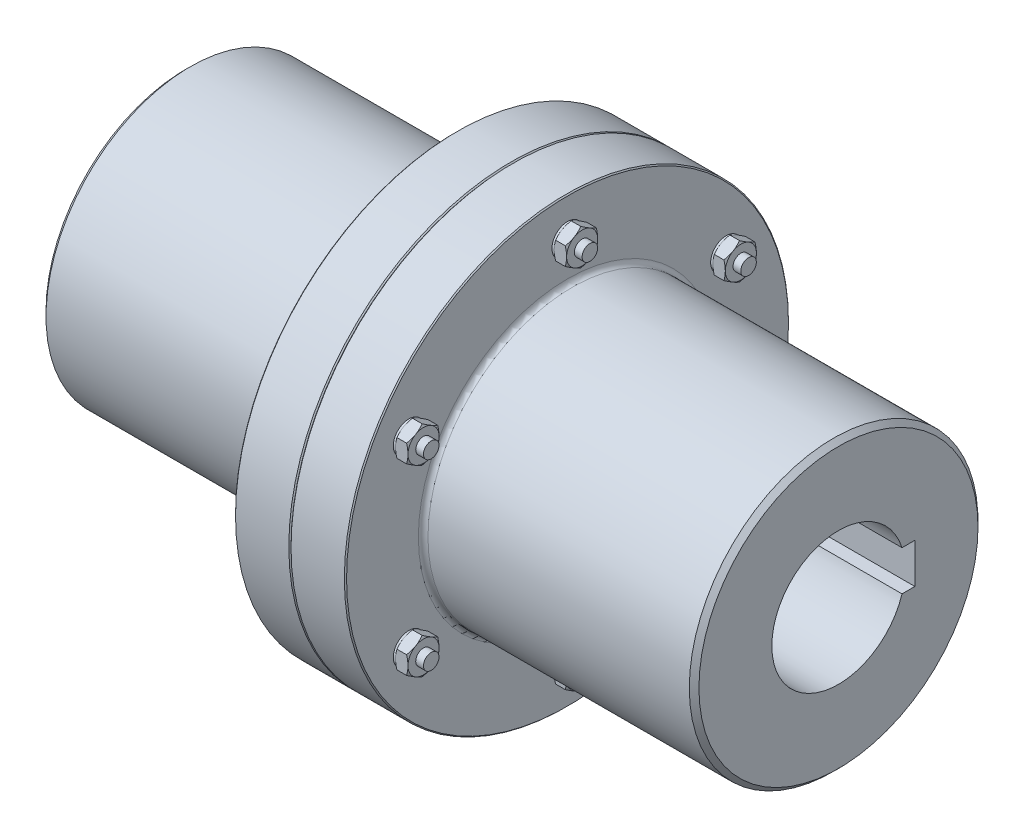
from build123d import *

# Parameters (mm, degrees)
CHAMFER1_SIZE                  = 2.166666667
CHAMFER2_SIZE                  = 0.5
FILLET1_R                      = 1
SKETCH15_R                     = 37.5
CUT_EXTRUDE5_DEPTH             = 204.982842416
CUT_EXTRUDE7_DEPTH             = 204.982842416
SKETCH16_R                     = 30
CUT_EXTRUDE6_DEPTH             = 204.982842416
CUT_EXTRUDE10_DEPTH            = 204.982842416
CHAMFER3_SIZE                  = 0.5
CHAMFER4_SIZE                  = 2.166666667
FILLET2_R                      = 2.166666667
SKETCH6_R                      = 3.5
CUT_EXTRUDE1_DEPTH             = 50
CHAMFER5_SIZE                  = 0.2
CHAMFER6_SIZE                  = 0.2
CIRPATTERN1_COUNT              = 6
CHAMFER5_OF_CIRPATTERN1_SIZE   = 0.2
CHAMFER6_OF_CIRPATTERN1_SIZE   = 0.2
SKETCH7_W                      = 60.08
SKETCH7_H                      = 3.5
BOSS_EXTRUDE1_DEPTH            = 5.6
SKETCH9_R                      = 10.5
SKETCH9_R_2                    = 7
CUT_EXTRUDE2_DEPTH             = 1
CUT_EXTRUDE2_DRAFT             = -60
SKETCH10_R                     = 7
BOSS_EXTRUDE2_DEPTH            = 1
BOSS_EXTRUDE3_DEPTH            = 5.6
SKETCH12_R                     = 10.5
SKETCH12_R_2                   = 7
CUT_EXTRUDE3_DEPTH             = 1
CUT_EXTRUDE3_DRAFT             = -60
SKETCH13_R                     = 10.5
SKETCH13_R_2                   = 7
CUT_EXTRUDE4_DEPTH             = 1
CUT_EXTRUDE4_DRAFT             = -60
CIRPATTERN3_COUNT              = 6
CIRPATTERN3_COPY_1_SKETCH_R    = 10.5
CIRPATTERN3_COPY_1_SKETCH_R_2  = 7
CIRPATTERN3_COPY_1_DEPTH       = 1
CIRPATTERN3_COPY_1_DRAFT       = -60
CIRPATTERN3_COPY_2_SKETCH_R    = 10.5
CIRPATTERN3_COPY_2_SKETCH_R_2  = 7
CIRPATTERN3_COPY_2_DEPTH       = 1
CIRPATTERN3_COPY_2_DRAFT       = -60
CIRPATTERN3_COPY_3_SKETCH_R    = 10.5
CIRPATTERN3_COPY_3_SKETCH_R_2  = 7
CIRPATTERN3_COPY_3_DEPTH       = 1
CIRPATTERN3_COPY_3_DRAFT       = -60
CIRPATTERN3_COPY_4_SKETCH_R    = 10.5
CIRPATTERN3_COPY_4_SKETCH_R_2  = 7
CIRPATTERN3_COPY_4_DEPTH       = 1
CIRPATTERN3_COPY_4_DRAFT       = -60
CIRPATTERN3_COPY_5_SKETCH_R    = 10.5
CIRPATTERN3_COPY_5_SKETCH_R_2  = 7
CIRPATTERN3_COPY_5_DEPTH       = 1
CIRPATTERN3_COPY_5_DRAFT       = -60
CIRPATTERN3_COPY_6_SKETCH_R    = 10.5
CIRPATTERN3_COPY_6_SKETCH_R_2  = 7
CIRPATTERN3_COPY_6_DEPTH       = 1
CIRPATTERN3_COPY_6_DRAFT       = -60
CIRPATTERN3_COPY_7_SKETCH_R    = 10.5
CIRPATTERN3_COPY_7_SKETCH_R_2  = 7
CIRPATTERN3_COPY_7_DEPTH       = 1
CIRPATTERN3_COPY_7_DRAFT       = -60
CIRPATTERN3_COPY_8_SKETCH_R    = 10.5
CIRPATTERN3_COPY_8_SKETCH_R_2  = 7
CIRPATTERN3_COPY_8_DEPTH       = 1
CIRPATTERN3_COPY_8_DRAFT       = -60
CIRPATTERN3_COPY_9_SKETCH_R    = 10.5
CIRPATTERN3_COPY_9_SKETCH_R_2  = 7
CIRPATTERN3_COPY_9_DEPTH       = 1
CIRPATTERN3_COPY_9_DRAFT       = -60
CIRPATTERN3_COPY_10_SKETCH_R   = 10.5
CIRPATTERN3_COPY_10_SKETCH_R_2 = 7
CIRPATTERN3_COPY_10_DEPTH      = 1
CIRPATTERN3_COPY_10_DRAFT      = -60
CIRPATTERN3_COPY_11_SKETCH_R   = 10.5
CIRPATTERN3_COPY_11_SKETCH_R_2 = 7
CIRPATTERN3_COPY_11_DEPTH      = 1
CIRPATTERN3_COPY_11_DRAFT      = -60
CIRPATTERN3_COPY_12_SKETCH_R   = 10.5
CIRPATTERN3_COPY_12_SKETCH_R_2 = 7
CIRPATTERN3_COPY_12_DEPTH      = 1
CIRPATTERN3_COPY_12_DRAFT      = -60
CIRPATTERN3_COPY_13_SKETCH_R   = 10.5
CIRPATTERN3_COPY_13_SKETCH_R_2 = 7
CIRPATTERN3_COPY_13_DEPTH      = 1
CIRPATTERN3_COPY_13_DRAFT      = -60
CIRPATTERN3_COPY_14_SKETCH_R   = 10.5
CIRPATTERN3_COPY_14_SKETCH_R_2 = 7
CIRPATTERN3_COPY_14_DEPTH      = 1
CIRPATTERN3_COPY_14_DRAFT      = -60
CIRPATTERN3_COPY_15_SKETCH_R   = 10.5
CIRPATTERN3_COPY_15_SKETCH_R_2 = 7
CIRPATTERN3_COPY_15_DEPTH      = 1
CIRPATTERN3_COPY_15_DRAFT      = -60


with BuildPart() as part:
    # Sketch2 → Revolve1 (revolve)
    with BuildSketch(Plane.XY, mode=Mode.PRIVATE) as revolve1_sk:
        Polygon((-147, 65), (-147, 0), (-5, 0), (-5, 70), (0, 70), (0, 100), (-25, 100), (-25, 65), align=None)
    revolve(revolve1_sk.sketch.rotate(Axis((-147, 0, 0), (1, 0, 0)), 90), axis=Axis((-147, 0, 0), (1, 0, 0)))

    # Chamfer1
    chamfer1_edges = [part.edges().sort_by_distance(p)[0] for p in [
        (-147, 0, -65),
    ]]
    chamfer(chamfer1_edges, length=CHAMFER1_SIZE)

    # Chamfer2
    chamfer2_edges = [part.edges().sort_by_distance(p)[0] for p in [
        (-25, 0, -100),
        (0, 0, -100),
    ]]
    chamfer(chamfer2_edges, length=CHAMFER2_SIZE)

    # Fillet1
    fillet1_edges = [part.edges().sort_by_distance(p)[0] for p in [
        (-25, 0, -65),
    ]]
    fillet(fillet1_edges, radius=FILLET1_R)

    # Sketch15 → Cut-Extrude5 (cut, through all)
    with BuildSketch(Plane(origin=(0, 0, 0), x_dir=(0, 0, -1), z_dir=(1, 0, 0))):
        Circle(SKETCH15_R)
    extrude(amount=-CUT_EXTRUDE5_DEPTH, mode=Mode.SUBTRACT)

    # Sketch20 → Cut-Extrude7 (cut, through all)
    with BuildSketch(Plane(origin=(0, 0, 0), x_dir=(0, 0, -1), z_dir=(1, 0, 0))):
        with BuildLine():
            Line((42.4, -10), (42.4, 10))
            Line((42.4, 10), (36.142080737, 10))
            ThreePointArc((36.142080737, 10), (37.158969493, 5.045888047), (37.5, 0))
            ThreePointArc((37.5, 0), (37.158969493, -5.045888047), (36.142080737, -10))
            Line((36.142080737, -10), (42.4, -10))
        make_face()
    extrude(amount=-CUT_EXTRUDE7_DEPTH, mode=Mode.SUBTRACT)


with BuildPart() as body_2:
    # Sketch3 → Revolve2 (revolve)
    with BuildSketch(Plane.XY, mode=Mode.PRIVATE) as revolve2_sk:
        Polygon((25, 100), (0, 100), (0, 70), (5, 70), (5, 0), (147, 0), (147, 30), (147, 65), (25, 65), align=None)
    revolve(revolve2_sk.sketch.rotate(Axis((-147, 0, 0), (1, 0, 0)), 270), axis=Axis((-147, 0, 0), (1, 0, 0)))

    # Sketch16 → Cut-Extrude6 (cut, through all)
    with BuildSketch(Plane(origin=(0, 0, 0), x_dir=(0, 0, -1), z_dir=(1, 0, 0))):
        Circle(SKETCH16_R)
    extrude(amount=CUT_EXTRUDE6_DEPTH, mode=Mode.SUBTRACT)

    # Sketch24 → Cut-Extrude10 (cut, through all)
    with BuildSketch(Plane(origin=(0, 0, 0), x_dir=(0, 0, -1), z_dir=(1, 0, 0))):
        with BuildLine():
            Line((34.4, -9), (34.4, 9))
            Line((34.4, 9), (28.618176043, 9))
            ThreePointArc((28.618176043, 9), (29.652531774, 4.552730978), (30, 0))
            ThreePointArc((30, 0), (29.652531774, -4.552730978), (28.618176043, -9))
            Line((28.618176043, -9), (34.4, -9))
        make_face()
    extrude(amount=CUT_EXTRUDE10_DEPTH, mode=Mode.SUBTRACT)

    # Chamfer3
    chamfer3_edges = [body_2.edges().sort_by_distance(p)[0] for p in [
        (25, 0, 100),
        (0, 0, 100),
    ]]
    chamfer(chamfer3_edges, length=CHAMFER3_SIZE)

    # Chamfer4
    chamfer4_edges = [body_2.edges().sort_by_distance(p)[0] for p in [
        (147, 0, 65),
    ]]
    chamfer(chamfer4_edges, length=CHAMFER4_SIZE)

    # Fillet2
    fillet2_edges = [body_2.edges().sort_by_distance(p)[0] for p in [
        (25, 0, 65),
    ]]
    fillet(fillet2_edges, radius=FILLET2_R)


with BuildPart() as cut_extrude1_tool:
    # Sketch6 → Cut-Extrude1 (new body)
    with BuildSketch(Plane.ZY.offset(25)):
        with Locations((0, 82.5)):
            Circle(SKETCH6_R)
    cut_extrude1 = extrude(amount=-CUT_EXTRUDE1_DEPTH)


with BuildPart() as part_1:
    add(part.part)

    # Cut-Extrude1: cut by cut_extrude1_tool
    add(cut_extrude1_tool.part, mode=Mode.SUBTRACT)

    # Chamfer5
    chamfer5_edges = [part_1.edges().sort_by_distance(p)[0] for p in [
        (-25, 82.5, -3.5),
    ]]
    chamfer(chamfer5_edges, length=CHAMFER5_SIZE)


with BuildPart() as body_2_1:
    add(body_2.part)

    # Cut-Extrude1: cut by cut_extrude1_tool
    add(cut_extrude1_tool.part, mode=Mode.SUBTRACT)

    # Chamfer6
    chamfer6_edges = [body_2_1.edges().sort_by_distance(p)[0] for p in [
        (25, 82.5, -3.5),
    ]]
    chamfer(chamfer6_edges, length=CHAMFER6_SIZE)


with BuildPart() as cirpattern1_tool:
    # CirPattern1: Cut-Extrude1 ×6 about axis
    cirpattern1_axis = Axis((0, 0, 0), (1, 0, 0))
    for i in range(1, CIRPATTERN1_COUNT):
        add(cut_extrude1.rotate(cirpattern1_axis, i * 360 / CIRPATTERN1_COUNT))


with BuildPart() as part_2:
    add(part_1.part)

    # CirPattern1: cut by cirpattern1_tool
    add(cirpattern1_tool.part, mode=Mode.SUBTRACT)

    # Chamfer5 of CirPattern1
    chamfer5_of_cirpattern1_edges = [part_2.edges().sort_by_distance(p)[0] for p in [
        (-25, 44.281088913, 69.697095812),
        (-25, -38.218911087, 73.197095812),
        (-25, -82.5, 3.5),
        (-25, -44.281088913, -69.697095812),
        (-25, 38.218911087, -73.197095812),
    ]]
    chamfer(chamfer5_of_cirpattern1_edges, length=CHAMFER5_OF_CIRPATTERN1_SIZE)



with BuildPart() as body_2_2:
    add(body_2_1.part)

    # CirPattern1: cut by cirpattern1_tool
    add(cirpattern1_tool.part, mode=Mode.SUBTRACT)

    # Chamfer6 of CirPattern1
    chamfer6_of_cirpattern1_edges = [body_2_2.edges().sort_by_distance(p)[0] for p in [
        (25, 44.281088913, 69.697095812),
        (25, -38.218911087, 73.197095812),
        (25, -82.5, 3.5),
        (25, -44.281088913, -69.697095812),
        (25, 38.218911087, -73.197095812),
    ]]
    chamfer(chamfer6_of_cirpattern1_edges, length=CHAMFER6_OF_CIRPATTERN1_SIZE)


with BuildPart() as part_3:
    add(part_2.part)

    add(body_2_2.part)  # Revolve3 merges body 2
    # Sketch7 → Revolve3 (revolve)
    with BuildSketch(Plane.XY, mode=Mode.PRIVATE) as revolve3_sk:
        with Locations((5.04, 84.25)):
            Rectangle(SKETCH7_W, SKETCH7_H)
    revolve3 = revolve(revolve3_sk.sketch.rotate(Axis((35.08, 82.5, 0), (-1, 0, 0)), 90), axis=Axis((35.08, 82.5, 0), (-1, 0, 0)))

    # Sketch8 → Boss-Extrude1 (add)
    with BuildSketch(Plane.ZY.offset(25)):
        Polygon((0, 90.582903769), (-7, 86.541451884), (-7, 78.458548116), (0, 74.417096231), (7, 78.458548116), (7, 86.541451884), align=None)
    boss_extrude1 = extrude(amount=BOSS_EXTRUDE1_DEPTH)


with BuildPart() as cut_extrude2_tool:
    # Sketch9 → Cut-Extrude2 (with draft: the straight prism first)
    with BuildSketch(Plane.ZY.offset(30.6)):
        with Locations((0, 82.5)):
            Circle(SKETCH9_R)
        with Locations((0, 82.5)):
            Circle(SKETCH9_R_2, mode=Mode.SUBTRACT)
    extrude(amount=-CUT_EXTRUDE2_DEPTH)
    # Cut-Extrude2: the draft: its side faces are tilted about the plane it starts from
    cut_extrude2_sides = [cut_extrude2_tool.faces().sort_by_distance(p)[0] for p in [
        (-30.1, 82.5, -10.5),
        (-30.1, 82.5, -7),
    ]]
    draft(cut_extrude2_sides, Plane.ZY.offset(30.6), CUT_EXTRUDE2_DRAFT)


with BuildPart() as part_4:
    add(part_3.part)

    # Cut-Extrude2: cut by cut_extrude2_tool
    add(cut_extrude2_tool.part, mode=Mode.SUBTRACT)

    # Sketch10 → Boss-Extrude2 (add)
    with BuildSketch(Plane(origin=(25, 0, 0), x_dir=(0, 0, -1), z_dir=(1, 0, 0))):
        with Locations(Location((0, 82.5, 0), (0, 0, 180))):
            Circle(SKETCH10_R)
    boss_extrude2 = extrude(amount=BOSS_EXTRUDE2_DEPTH)

    # Sketch11 → Boss-Extrude3 (add)
    with BuildSketch(Plane(origin=(26, 0, 0), x_dir=(0, 0, -1), z_dir=(1, 0, 0))):
        Polygon((7, 86.541451884), (0, 90.582903769), (-7, 86.541451884), (-7, 78.458548116), (0, 74.417096231), (7, 78.458548116), align=None)
    boss_extrude3 = extrude(amount=BOSS_EXTRUDE3_DEPTH)


with BuildPart() as cut_extrude3_tool:
    # Sketch12 → Cut-Extrude3 (with draft: the straight prism first)
    with BuildSketch(Plane(origin=(31.6, 0, 0), x_dir=(0, 0, -1), z_dir=(1, 0, 0))):
        with Locations((0, 82.5)):
            Circle(SKETCH12_R)
        with Locations(Location((0, 82.5, 0), (0, 0, 180))):
            Circle(SKETCH12_R_2, mode=Mode.SUBTRACT)
    extrude(amount=-CUT_EXTRUDE3_DEPTH)
    # Cut-Extrude3: the draft: its side faces are tilted about the plane it starts from
    cut_extrude3_sides = [cut_extrude3_tool.faces().sort_by_distance(p)[0] for p in [
        (31.1, 82.5, 10.5),
        (31.1, 82.5, -7),
    ]]
    draft(cut_extrude3_sides, Plane(origin=(31.6, 0, 0), x_dir=(0, 0, -1), z_dir=(1, 0, 0)), CUT_EXTRUDE3_DRAFT)


with BuildPart() as part_5:
    add(part_4.part)

    # Cut-Extrude3: cut by cut_extrude3_tool
    add(cut_extrude3_tool.part, mode=Mode.SUBTRACT)


with BuildPart() as cut_extrude4_tool:
    # Sketch13 → Cut-Extrude4 (with draft: the straight prism first)
    with BuildSketch(Plane.ZY.offset(-26)):
        with Locations((0, 82.5)):
            Circle(SKETCH13_R)
        with Locations((0, 82.5)):
            Circle(SKETCH13_R_2, mode=Mode.SUBTRACT)
    extrude(amount=-CUT_EXTRUDE4_DEPTH)
    # Cut-Extrude4: the draft: its side faces are tilted about the plane it starts from
    cut_extrude4_sides = [cut_extrude4_tool.faces().sort_by_distance(p)[0] for p in [
        (26.5, 82.5, -10.5),
        (26.5, 82.5, -7),
    ]]
    draft(cut_extrude4_sides, Plane.ZY.offset(-26), CUT_EXTRUDE4_DRAFT)


with BuildPart() as part_6:
    add(part_5.part)

    # Cut-Extrude4: cut by cut_extrude4_tool
    add(cut_extrude4_tool.part, mode=Mode.SUBTRACT)

    # CirPattern3: Revolve3, Boss-Extrude1, Boss-Extrude2, Boss-Extrude3 ×6 about axis
    cirpattern3_axis = Axis((0, 0, 0), (1, 0, 0))
    add([revolve3.rotate(cirpattern3_axis, i * 360 / CIRPATTERN3_COUNT) for i in range(1, CIRPATTERN3_COUNT)])
    add([boss_extrude1.rotate(cirpattern3_axis, i * 360 / CIRPATTERN3_COUNT) for i in range(1, CIRPATTERN3_COUNT)])
    add([boss_extrude2.rotate(cirpattern3_axis, i * 360 / CIRPATTERN3_COUNT) for i in range(1, CIRPATTERN3_COUNT)])
    add([boss_extrude3.rotate(cirpattern3_axis, i * 360 / CIRPATTERN3_COUNT) for i in range(1, CIRPATTERN3_COUNT)])


with BuildPart() as cirpattern3_copy_1_tool:
    # CirPattern3 copy 1 sketch → CirPattern3 copy 1 (with draft: the straight prism first)
    with BuildSketch(Plane(origin=(-30.6, 0, 0), x_dir=(0, -0.8660254037844386, 0.5000000000000001), z_dir=(-1, 0, 0))):
        with Locations((0, 82.5)):
            Circle(CIRPATTERN3_COPY_1_SKETCH_R)
        with Locations((0, 82.5)):
            Circle(CIRPATTERN3_COPY_1_SKETCH_R_2, mode=Mode.SUBTRACT)
    extrude(amount=-CIRPATTERN3_COPY_1_DEPTH)
    # CirPattern3 copy 1: the draft: its side faces are tilted about the plane it starts from
    cirpattern3_copy_1_sides = [cirpattern3_copy_1_tool.faces().sort_by_distance(p)[0] for p in [
        (-30.1, 50.34326674, 66.197095812),
        (-30.1, 47.312177826, 67.947095812),
    ]]
    draft(cirpattern3_copy_1_sides, Plane(origin=(-30.6, 0, 0), x_dir=(0, -0.8660254037844386, 0.5000000000000001), z_dir=(-1, 0, 0)), CIRPATTERN3_COPY_1_DRAFT)


with BuildPart() as part_7:
    add(part_6.part)

    # CirPattern3 copy 1: cut by cirpattern3_copy_1_tool
    add(cirpattern3_copy_1_tool.part, mode=Mode.SUBTRACT)


with BuildPart() as cirpattern3_copy_2_tool:
    # CirPattern3 copy 2 sketch → CirPattern3 copy 2 (with draft: the straight prism first)
    with BuildSketch(Plane(origin=(-30.6, 0, 0), x_dir=(0, -0.8660254037844387, -0.4999999999999998), z_dir=(-1, 0, 0))):
        with Locations((0, 82.5)):
            Circle(CIRPATTERN3_COPY_2_SKETCH_R)
        with Locations((0, 82.5)):
            Circle(CIRPATTERN3_COPY_2_SKETCH_R_2, mode=Mode.SUBTRACT)
    extrude(amount=-CIRPATTERN3_COPY_2_DEPTH)
    # CirPattern3 copy 2: the draft: its side faces are tilted about the plane it starts from
    cirpattern3_copy_2_sides = [cirpattern3_copy_2_tool.faces().sort_by_distance(p)[0] for p in [
        (-30.1, -32.15673326, 76.697095812),
        (-30.1, -35.187822174, 74.947095812),
    ]]
    draft(cirpattern3_copy_2_sides, Plane(origin=(-30.6, 0, 0), x_dir=(0, -0.8660254037844387, -0.4999999999999998), z_dir=(-1, 0, 0)), CIRPATTERN3_COPY_2_DRAFT)


with BuildPart() as part_8:
    add(part_7.part)

    # CirPattern3 copy 2: cut by cirpattern3_copy_2_tool
    add(cirpattern3_copy_2_tool.part, mode=Mode.SUBTRACT)


with BuildPart() as cirpattern3_copy_3_tool:
    # CirPattern3 copy 3 sketch → CirPattern3 copy 3 (with draft: the straight prism first)
    with BuildSketch(Plane(origin=(-30.6, 0, 0), x_dir=(0, 0, -1), z_dir=(-1, 0, 0))):
        with Locations((0, 82.5)):
            Circle(CIRPATTERN3_COPY_3_SKETCH_R)
        with Locations((0, 82.5)):
            Circle(CIRPATTERN3_COPY_3_SKETCH_R_2, mode=Mode.SUBTRACT)
    extrude(amount=-CIRPATTERN3_COPY_3_DEPTH)
    # CirPattern3 copy 3: the draft: its side faces are tilted about the plane it starts from
    cirpattern3_copy_3_sides = [cirpattern3_copy_3_tool.faces().sort_by_distance(p)[0] for p in [
        (-30.1, -82.5, 10.5),
        (-30.1, -82.5, 7),
    ]]
    draft(cirpattern3_copy_3_sides, Plane(origin=(-30.6, 0, 0), x_dir=(0, 0, -1), z_dir=(-1, 0, 0)), CIRPATTERN3_COPY_3_DRAFT)


with BuildPart() as part_9:
    add(part_8.part)

    # CirPattern3 copy 3: cut by cirpattern3_copy_3_tool
    add(cirpattern3_copy_3_tool.part, mode=Mode.SUBTRACT)


with BuildPart() as cirpattern3_copy_4_tool:
    # CirPattern3 copy 4 sketch → CirPattern3 copy 4 (with draft: the straight prism first)
    with BuildSketch(Plane(origin=(-30.6, 0, 0), x_dir=(0, 0.8660254037844384, -0.5000000000000004), z_dir=(-1, 0, 0))):
        with Locations((0, 82.5)):
            Circle(CIRPATTERN3_COPY_4_SKETCH_R)
        with Locations((0, 82.5)):
            Circle(CIRPATTERN3_COPY_4_SKETCH_R_2, mode=Mode.SUBTRACT)
    extrude(amount=-CIRPATTERN3_COPY_4_DEPTH)
    # CirPattern3 copy 4: the draft: its side faces are tilted about the plane it starts from
    cirpattern3_copy_4_sides = [cirpattern3_copy_4_tool.faces().sort_by_distance(p)[0] for p in [
        (-30.1, -50.34326674, -66.197095812),
        (-30.1, -47.312177826, -67.947095812),
    ]]
    draft(cirpattern3_copy_4_sides, Plane(origin=(-30.6, 0, 0), x_dir=(0, 0.8660254037844384, -0.5000000000000004), z_dir=(-1, 0, 0)), CIRPATTERN3_COPY_4_DRAFT)


with BuildPart() as part_10:
    add(part_9.part)

    # CirPattern3 copy 4: cut by cirpattern3_copy_4_tool
    add(cirpattern3_copy_4_tool.part, mode=Mode.SUBTRACT)


with BuildPart() as cirpattern3_copy_5_tool:
    # CirPattern3 copy 5 sketch → CirPattern3 copy 5 (with draft: the straight prism first)
    with BuildSketch(Plane(origin=(-30.6, 0, 0), x_dir=(0, 0.8660254037844386, 0.5000000000000001), z_dir=(-1, 0, 0))):
        with Locations((0, 82.5)):
            Circle(CIRPATTERN3_COPY_5_SKETCH_R)
        with Locations((0, 82.5)):
            Circle(CIRPATTERN3_COPY_5_SKETCH_R_2, mode=Mode.SUBTRACT)
    extrude(amount=-CIRPATTERN3_COPY_5_DEPTH)
    # CirPattern3 copy 5: the draft: its side faces are tilted about the plane it starts from
    cirpattern3_copy_5_sides = [cirpattern3_copy_5_tool.faces().sort_by_distance(p)[0] for p in [
        (-30.1, 32.15673326, -76.697095812),
        (-30.1, 35.187822174, -74.947095812),
    ]]
    draft(cirpattern3_copy_5_sides, Plane(origin=(-30.6, 0, 0), x_dir=(0, 0.8660254037844386, 0.5000000000000001), z_dir=(-1, 0, 0)), CIRPATTERN3_COPY_5_DRAFT)


with BuildPart() as part_11:
    add(part_10.part)

    # CirPattern3 copy 5: cut by cirpattern3_copy_5_tool
    add(cirpattern3_copy_5_tool.part, mode=Mode.SUBTRACT)


with BuildPart() as cirpattern3_copy_6_tool:
    # CirPattern3 copy 6 sketch → CirPattern3 copy 6 (with draft: the straight prism first)
    with BuildSketch(Plane(origin=(31.6, 0, 0), x_dir=(0, 0.8660254037844386, -0.5000000000000001), z_dir=(1, 0, 0))):
        with Locations((0, 82.5)):
            Circle(CIRPATTERN3_COPY_6_SKETCH_R)
        with Locations(Location((0, 82.5, 0), (0, 0, 180))):
            Circle(CIRPATTERN3_COPY_6_SKETCH_R_2, mode=Mode.SUBTRACT)
    extrude(amount=-CIRPATTERN3_COPY_6_DEPTH)
    # CirPattern3 copy 6: the draft: its side faces are tilted about the plane it starts from
    cirpattern3_copy_6_sides = [cirpattern3_copy_6_tool.faces().sort_by_distance(p)[0] for p in [
        (31.1, 32.15673326, 76.697095812),
        (31.1, 47.312177826, 67.947095812),
    ]]
    draft(cirpattern3_copy_6_sides, Plane(origin=(31.6, 0, 0), x_dir=(0, 0.8660254037844386, -0.5000000000000001), z_dir=(1, 0, 0)), CIRPATTERN3_COPY_6_DRAFT)


with BuildPart() as part_12:
    add(part_11.part)

    # CirPattern3 copy 6: cut by cirpattern3_copy_6_tool
    add(cirpattern3_copy_6_tool.part, mode=Mode.SUBTRACT)


with BuildPart() as cirpattern3_copy_7_tool:
    # CirPattern3 copy 7 sketch → CirPattern3 copy 7 (with draft: the straight prism first)
    with BuildSketch(Plane(origin=(31.6, 0, 0), x_dir=(0, 0.8660254037844387, 0.4999999999999998), z_dir=(1, 0, 0))):
        with Locations((0, 82.5)):
            Circle(CIRPATTERN3_COPY_7_SKETCH_R)
        with Locations(Location((0, 82.5, 0), (0, 0, 180))):
            Circle(CIRPATTERN3_COPY_7_SKETCH_R_2, mode=Mode.SUBTRACT)
    extrude(amount=-CIRPATTERN3_COPY_7_DEPTH)
    # CirPattern3 copy 7: the draft: its side faces are tilted about the plane it starts from
    cirpattern3_copy_7_sides = [cirpattern3_copy_7_tool.faces().sort_by_distance(p)[0] for p in [
        (31.1, -50.34326674, 66.197095812),
        (31.1, -35.187822174, 74.947095812),
    ]]
    draft(cirpattern3_copy_7_sides, Plane(origin=(31.6, 0, 0), x_dir=(0, 0.8660254037844387, 0.4999999999999998), z_dir=(1, 0, 0)), CIRPATTERN3_COPY_7_DRAFT)


with BuildPart() as part_13:
    add(part_12.part)

    # CirPattern3 copy 7: cut by cirpattern3_copy_7_tool
    add(cirpattern3_copy_7_tool.part, mode=Mode.SUBTRACT)


with BuildPart() as cirpattern3_copy_8_tool:
    # CirPattern3 copy 8 sketch → CirPattern3 copy 8 (with draft: the straight prism first)
    with BuildSketch(Plane(origin=(31.6, 0, 0), x_dir=(0, 0, 1), z_dir=(1, 0, 0))):
        with Locations((0, 82.5)):
            Circle(CIRPATTERN3_COPY_8_SKETCH_R)
        with Locations(Location((0, 82.5, 0), (0, 0, 180))):
            Circle(CIRPATTERN3_COPY_8_SKETCH_R_2, mode=Mode.SUBTRACT)
    extrude(amount=-CIRPATTERN3_COPY_8_DEPTH)
    # CirPattern3 copy 8: the draft: its side faces are tilted about the plane it starts from
    cirpattern3_copy_8_sides = [cirpattern3_copy_8_tool.faces().sort_by_distance(p)[0] for p in [
        (31.1, -82.5, -10.5),
        (31.1, -82.5, 7),
    ]]
    draft(cirpattern3_copy_8_sides, Plane(origin=(31.6, 0, 0), x_dir=(0, 0, 1), z_dir=(1, 0, 0)), CIRPATTERN3_COPY_8_DRAFT)


with BuildPart() as part_14:
    add(part_13.part)

    # CirPattern3 copy 8: cut by cirpattern3_copy_8_tool
    add(cirpattern3_copy_8_tool.part, mode=Mode.SUBTRACT)


with BuildPart() as cirpattern3_copy_9_tool:
    # CirPattern3 copy 9 sketch → CirPattern3 copy 9 (with draft: the straight prism first)
    with BuildSketch(Plane(origin=(31.6, 0, 0), x_dir=(0, -0.8660254037844384, 0.5000000000000004), z_dir=(1, 0, 0))):
        with Locations((0, 82.5)):
            Circle(CIRPATTERN3_COPY_9_SKETCH_R)
        with Locations(Location((0, 82.5, 0), (0, 0, 180))):
            Circle(CIRPATTERN3_COPY_9_SKETCH_R_2, mode=Mode.SUBTRACT)
    extrude(amount=-CIRPATTERN3_COPY_9_DEPTH)
    # CirPattern3 copy 9: the draft: its side faces are tilted about the plane it starts from
    cirpattern3_copy_9_sides = [cirpattern3_copy_9_tool.faces().sort_by_distance(p)[0] for p in [
        (31.1, -32.15673326, -76.697095812),
        (31.1, -47.312177826, -67.947095812),
    ]]
    draft(cirpattern3_copy_9_sides, Plane(origin=(31.6, 0, 0), x_dir=(0, -0.8660254037844384, 0.5000000000000004), z_dir=(1, 0, 0)), CIRPATTERN3_COPY_9_DRAFT)


with BuildPart() as part_15:
    add(part_14.part)

    # CirPattern3 copy 9: cut by cirpattern3_copy_9_tool
    add(cirpattern3_copy_9_tool.part, mode=Mode.SUBTRACT)


with BuildPart() as cirpattern3_copy_10_tool:
    # CirPattern3 copy 10 sketch → CirPattern3 copy 10 (with draft: the straight prism first)
    with BuildSketch(Plane(origin=(31.6, 0, 0), x_dir=(0, -0.8660254037844386, -0.5000000000000001), z_dir=(1, 0, 0))):
        with Locations((0, 82.5)):
            Circle(CIRPATTERN3_COPY_10_SKETCH_R)
        with Locations(Location((0, 82.5, 0), (0, 0, 180))):
            Circle(CIRPATTERN3_COPY_10_SKETCH_R_2, mode=Mode.SUBTRACT)
    extrude(amount=-CIRPATTERN3_COPY_10_DEPTH)
    # CirPattern3 copy 10: the draft: its side faces are tilted about the plane it starts from
    cirpattern3_copy_10_sides = [cirpattern3_copy_10_tool.faces().sort_by_distance(p)[0] for p in [
        (31.1, 50.34326674, -66.197095812),
        (31.1, 35.187822174, -74.947095812),
    ]]
    draft(cirpattern3_copy_10_sides, Plane(origin=(31.6, 0, 0), x_dir=(0, -0.8660254037844386, -0.5000000000000001), z_dir=(1, 0, 0)), CIRPATTERN3_COPY_10_DRAFT)


with BuildPart() as part_16:
    add(part_15.part)

    # CirPattern3 copy 10: cut by cirpattern3_copy_10_tool
    add(cirpattern3_copy_10_tool.part, mode=Mode.SUBTRACT)


with BuildPart() as cirpattern3_copy_11_tool:
    # CirPattern3 copy 11 sketch → CirPattern3 copy 11 (with draft: the straight prism first)
    with BuildSketch(Plane(origin=(26, 0, 0), x_dir=(0, -0.8660254037844386, 0.5000000000000001), z_dir=(-1, 0, 0))):
        with Locations((0, 82.5)):
            Circle(CIRPATTERN3_COPY_11_SKETCH_R)
        with Locations((0, 82.5)):
            Circle(CIRPATTERN3_COPY_11_SKETCH_R_2, mode=Mode.SUBTRACT)
    extrude(amount=-CIRPATTERN3_COPY_11_DEPTH)
    # CirPattern3 copy 11: the draft: its side faces are tilted about the plane it starts from
    cirpattern3_copy_11_sides = [cirpattern3_copy_11_tool.faces().sort_by_distance(p)[0] for p in [
        (26.5, 50.34326674, 66.197095812),
        (26.5, 47.312177826, 67.947095812),
    ]]
    draft(cirpattern3_copy_11_sides, Plane(origin=(26, 0, 0), x_dir=(0, -0.8660254037844386, 0.5000000000000001), z_dir=(-1, 0, 0)), CIRPATTERN3_COPY_11_DRAFT)


with BuildPart() as part_17:
    add(part_16.part)

    # CirPattern3 copy 11: cut by cirpattern3_copy_11_tool
    add(cirpattern3_copy_11_tool.part, mode=Mode.SUBTRACT)


with BuildPart() as cirpattern3_copy_12_tool:
    # CirPattern3 copy 12 sketch → CirPattern3 copy 12 (with draft: the straight prism first)
    with BuildSketch(Plane(origin=(26, 0, 0), x_dir=(0, -0.8660254037844387, -0.4999999999999998), z_dir=(-1, 0, 0))):
        with Locations((0, 82.5)):
            Circle(CIRPATTERN3_COPY_12_SKETCH_R)
        with Locations((0, 82.5)):
            Circle(CIRPATTERN3_COPY_12_SKETCH_R_2, mode=Mode.SUBTRACT)
    extrude(amount=-CIRPATTERN3_COPY_12_DEPTH)
    # CirPattern3 copy 12: the draft: its side faces are tilted about the plane it starts from
    cirpattern3_copy_12_sides = [cirpattern3_copy_12_tool.faces().sort_by_distance(p)[0] for p in [
        (26.5, -32.15673326, 76.697095812),
        (26.5, -35.187822174, 74.947095812),
    ]]
    draft(cirpattern3_copy_12_sides, Plane(origin=(26, 0, 0), x_dir=(0, -0.8660254037844387, -0.4999999999999998), z_dir=(-1, 0, 0)), CIRPATTERN3_COPY_12_DRAFT)


with BuildPart() as part_18:
    add(part_17.part)

    # CirPattern3 copy 12: cut by cirpattern3_copy_12_tool
    add(cirpattern3_copy_12_tool.part, mode=Mode.SUBTRACT)


with BuildPart() as cirpattern3_copy_13_tool:
    # CirPattern3 copy 13 sketch → CirPattern3 copy 13 (with draft: the straight prism first)
    with BuildSketch(Plane(origin=(26, 0, 0), x_dir=(0, 0, -1), z_dir=(-1, 0, 0))):
        with Locations((0, 82.5)):
            Circle(CIRPATTERN3_COPY_13_SKETCH_R)
        with Locations((0, 82.5)):
            Circle(CIRPATTERN3_COPY_13_SKETCH_R_2, mode=Mode.SUBTRACT)
    extrude(amount=-CIRPATTERN3_COPY_13_DEPTH)
    # CirPattern3 copy 13: the draft: its side faces are tilted about the plane it starts from
    cirpattern3_copy_13_sides = [cirpattern3_copy_13_tool.faces().sort_by_distance(p)[0] for p in [
        (26.5, -82.5, 10.5),
        (26.5, -82.5, 7),
    ]]
    draft(cirpattern3_copy_13_sides, Plane(origin=(26, 0, 0), x_dir=(0, 0, -1), z_dir=(-1, 0, 0)), CIRPATTERN3_COPY_13_DRAFT)


with BuildPart() as part_19:
    add(part_18.part)

    # CirPattern3 copy 13: cut by cirpattern3_copy_13_tool
    add(cirpattern3_copy_13_tool.part, mode=Mode.SUBTRACT)


with BuildPart() as cirpattern3_copy_14_tool:
    # CirPattern3 copy 14 sketch → CirPattern3 copy 14 (with draft: the straight prism first)
    with BuildSketch(Plane(origin=(26, 0, 0), x_dir=(0, 0.8660254037844384, -0.5000000000000004), z_dir=(-1, 0, 0))):
        with Locations((0, 82.5)):
            Circle(CIRPATTERN3_COPY_14_SKETCH_R)
        with Locations((0, 82.5)):
            Circle(CIRPATTERN3_COPY_14_SKETCH_R_2, mode=Mode.SUBTRACT)
    extrude(amount=-CIRPATTERN3_COPY_14_DEPTH)
    # CirPattern3 copy 14: the draft: its side faces are tilted about the plane it starts from
    cirpattern3_copy_14_sides = [cirpattern3_copy_14_tool.faces().sort_by_distance(p)[0] for p in [
        (26.5, -50.34326674, -66.197095812),
        (26.5, -47.312177826, -67.947095812),
    ]]
    draft(cirpattern3_copy_14_sides, Plane(origin=(26, 0, 0), x_dir=(0, 0.8660254037844384, -0.5000000000000004), z_dir=(-1, 0, 0)), CIRPATTERN3_COPY_14_DRAFT)


with BuildPart() as part_20:
    add(part_19.part)

    # CirPattern3 copy 14: cut by cirpattern3_copy_14_tool
    add(cirpattern3_copy_14_tool.part, mode=Mode.SUBTRACT)


with BuildPart() as cirpattern3_copy_15_tool:
    # CirPattern3 copy 15 sketch → CirPattern3 copy 15 (with draft: the straight prism first)
    with BuildSketch(Plane(origin=(26, 0, 0), x_dir=(0, 0.8660254037844386, 0.5000000000000001), z_dir=(-1, 0, 0))):
        with Locations((0, 82.5)):
            Circle(CIRPATTERN3_COPY_15_SKETCH_R)
        with Locations((0, 82.5)):
            Circle(CIRPATTERN3_COPY_15_SKETCH_R_2, mode=Mode.SUBTRACT)
    extrude(amount=-CIRPATTERN3_COPY_15_DEPTH)
    # CirPattern3 copy 15: the draft: its side faces are tilted about the plane it starts from
    cirpattern3_copy_15_sides = [cirpattern3_copy_15_tool.faces().sort_by_distance(p)[0] for p in [
        (26.5, 32.15673326, -76.697095812),
        (26.5, 35.187822174, -74.947095812),
    ]]
    draft(cirpattern3_copy_15_sides, Plane(origin=(26, 0, 0), x_dir=(0, 0.8660254037844386, 0.5000000000000001), z_dir=(-1, 0, 0)), CIRPATTERN3_COPY_15_DRAFT)


with BuildPart() as part_21:
    add(part_20.part)

    # CirPattern3 copy 15: cut by cirpattern3_copy_15_tool
    add(cirpattern3_copy_15_tool.part, mode=Mode.SUBTRACT)


solid = part_21.part
